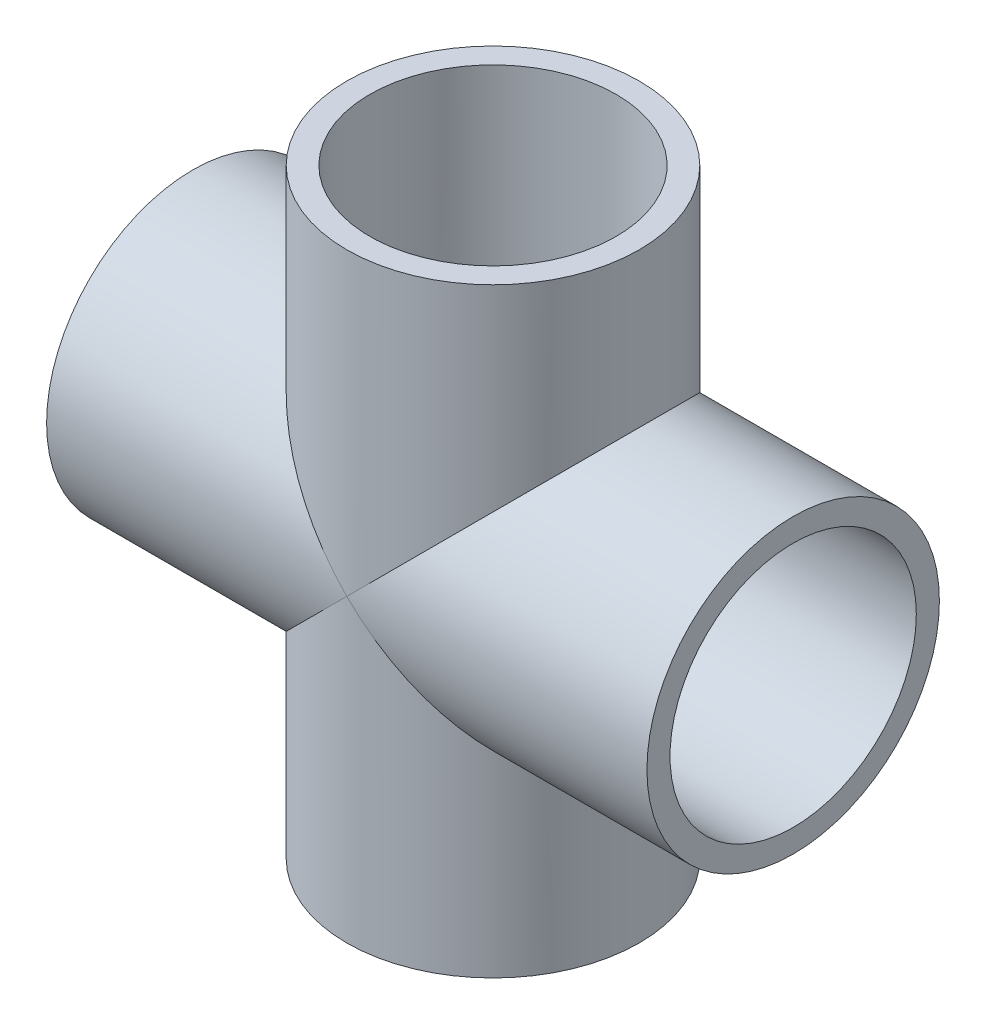
from build123d import *

# Parameters (mm, degrees)
SKETCH_1_W               = 3
SKETCH_1_H               = 39
PATTERN_CIRCULAR_1_COUNT = 4
SKETCH_5_R               = 16
CUT_EXTRUDE_1_DEPTH      = 90.252451078
SKETCH_6_R               = 16
CUT_EXTRUDE_2_DEPTH      = 90.252451078


with BuildPart() as part:
    # 草图1 → 旋转1 (revolve)
    with BuildSketch(Plane.XY, mode=Mode.PRIVATE) as revolve_1_sk:
        with Locations((-17.5, 19.5)):
            Rectangle(SKETCH_1_W, SKETCH_1_H)
    revolve_1 = revolve(revolve_1_sk.sketch.rotate(Axis((0, 0, 0), (0, 1, 0)), 270), axis=Axis((0, 0, 0), (0, 1, 0)))

    # 阵列(圆周)1: 旋转1 ×4 about axis
    pattern_circular_1_axis = Axis((0, 0, 0), (0, 0, 1))
    for i in range(1, PATTERN_CIRCULAR_1_COUNT):
        add(revolve_1.rotate(pattern_circular_1_axis, i * 360 / PATTERN_CIRCULAR_1_COUNT))

    # 草图5 → 切除-拉伸1 (cut, through all)
    with BuildSketch(Plane(origin=(0, 39, 0), x_dir=(1, 0, 0), z_dir=(0, 1, 0))):
        with Locations(Location((0, 0, 0), (0, 0, 90))):
            Circle(SKETCH_5_R)
    extrude(amount=-CUT_EXTRUDE_1_DEPTH, mode=Mode.SUBTRACT)

    # 草图6 → 切除-拉伸2 (cut, through all)
    with BuildSketch(Plane(origin=(39, 0, 0), x_dir=(0, 0, -1), z_dir=(1, 0, 0))):
        Circle(SKETCH_6_R)
    extrude(amount=-CUT_EXTRUDE_2_DEPTH, mode=Mode.SUBTRACT)


solid = part.part
